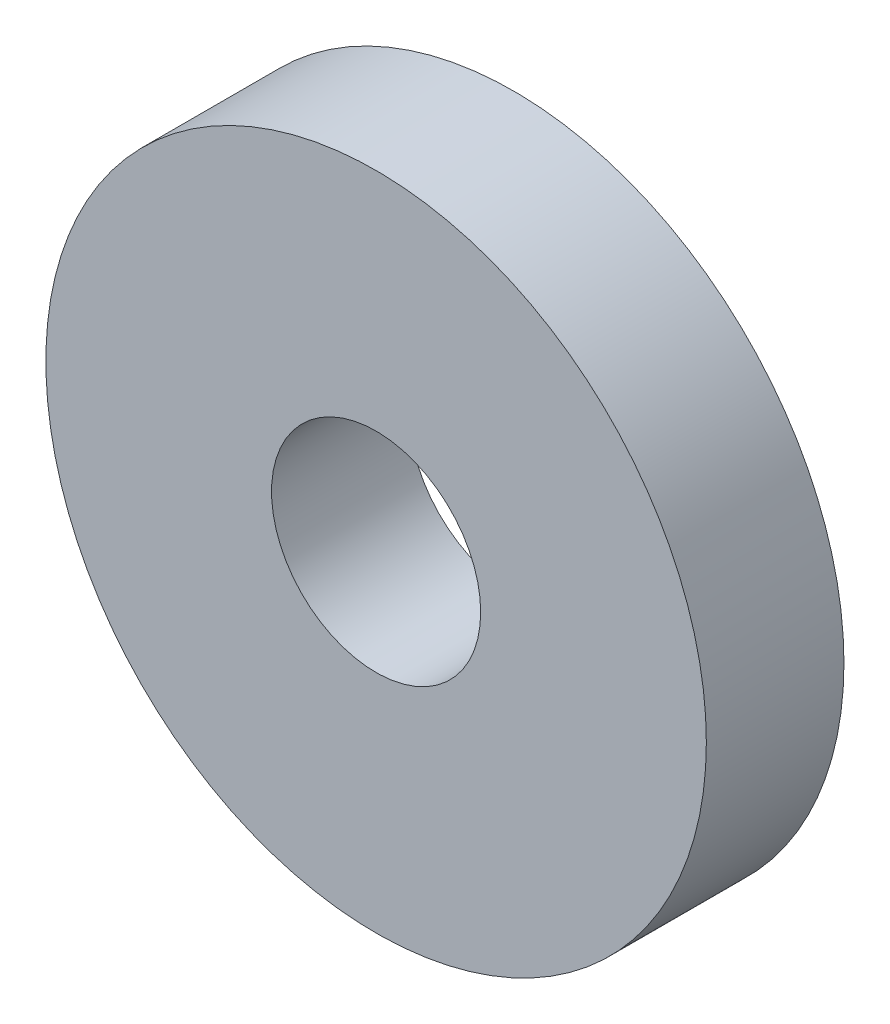
from build123d import *

# Parameters (mm, degrees)
SKETCH_1_R      = 7.6
EXTRUDE_1_DEPTH = 10


with BuildPart() as part:
    # 草图1 → 凸台-拉伸1 (new body)
    with BuildSketch(Plane.XY):
        with BuildLine():
            ThreePointArc((-23.972773672, -1.142857143), (0, -24), (23.972773672, -1.142857143))
            ThreePointArc((23.972773672, -1.142857143), (0, 24), (-23.972773672, -1.142857143))
        make_face()
        Circle(SKETCH_1_R, mode=Mode.SUBTRACT)
    extrude(amount=EXTRUDE_1_DEPTH)


solid = part.part
